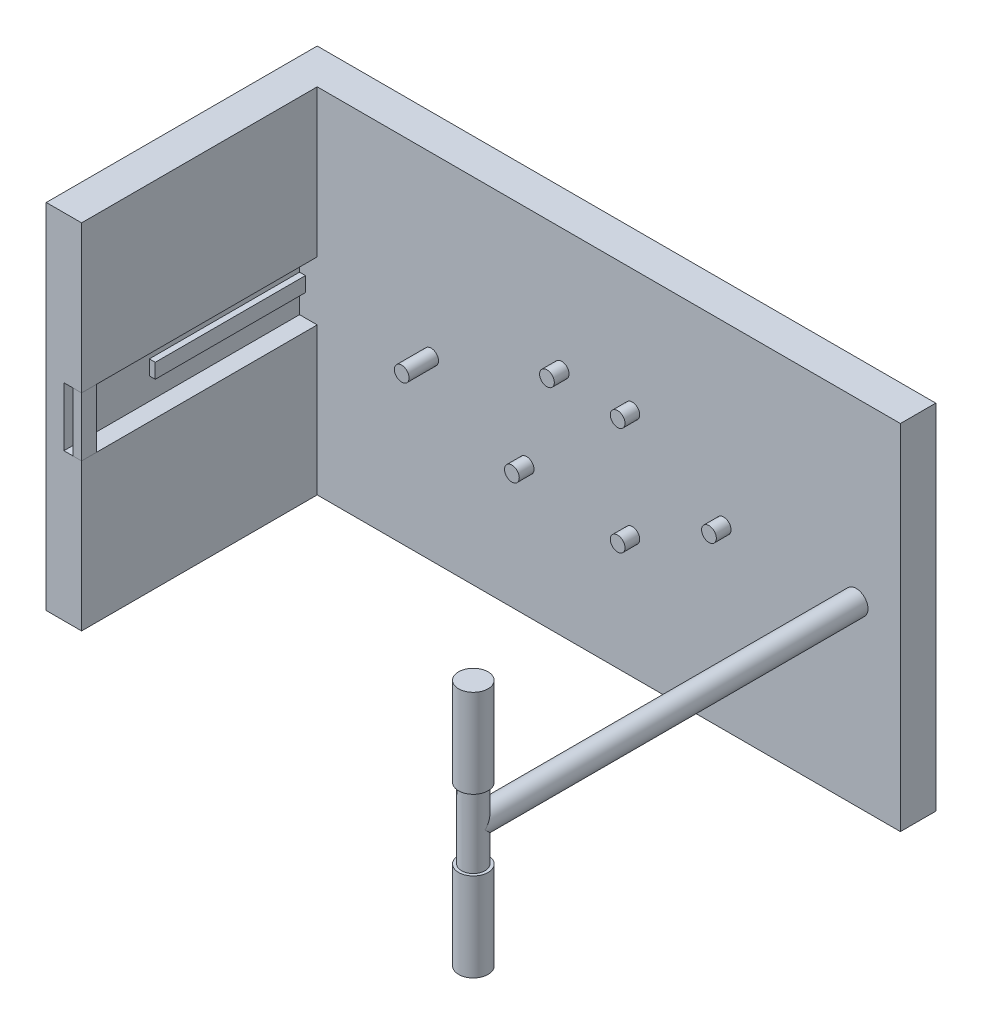
SolidWorks part; units mm, degrees
ref_plane "Front Plane" through (0, 0, 0) normal (0, 0, 1) x (1, 0, 0)
ref_plane "Top Plane" through (0, 0, 0) normal (0, 1, 0) x (1, 0, 0)
ref_plane "Right Plane" through (0, 0, 0) normal (1, 0, 0) x (0, 0, -1)
other "Configuration Table"
sketch "Sketch1" plane through (0, 0, 0) normal (0, 0, 1) x (1, 0, 0)
  line L0 (0, 3.2171) -> (0, -3.2171) construction
  point P4 (0, 0)
sketch "Sketch2" plane through (0, 0, 0) normal (0, 0, 1) x (1, 0, 0)
  line L1 (0, 0) -> (2100, 0)
  line L2 (0, 0) -> (0, -1200)
  line L3 (0, -1200) -> (2100, -1200)
  line L4 (2100, 0) -> (2100, -1200)
  dimension "D1" = 1200
  dimension "D2" = 2100
extrude "Boss-Extrude1" add sketch "Sketch2" along normal blind 120
sketch "Sketch3" plane through (0, 0, 120) normal (0, 0, 1) x (1, 0, 0)
  line L0 (0, -1200) -> (2100, -1200) construction
  line L1 (0, 0) -> (120, 0)
  line L2 (0, 0) -> (0, -1200)
  line L3 (0, -1200) -> (120, -1200)
  line L4 (120, 0) -> (120, -1200)
  dimension "D1" = 120
extrude "Boss-Extrude2" add sketch "Sketch3" along normal blind 800
sketch "Sketch4" plane through (0, 0, 120) normal (0, 0, 1) x (1, 0, 0)
  line L0 (1950, 0) -> (1950, -1200) construction
  line L1 (2100, 0) -> (120, 0) construction
  line L2 (120, -1200) -> (2100, -1200) construction
  line L3 (2100, -1200) -> (2100, 0) construction
  circle A0 centre (1950, -600) radius 40
  dimension "D2" = 80
  dimension "D1" = 150
extrude "Boss-Extrude3" add sketch "Sketch4" along normal blind 1300
sketch "Sketch5" plane through (0, 0, 1420) normal (0, 0, 1) x (1, 0, 0)
  line L0 (1950, -560) -> (1950, -640)
  line L1 (1990, -600) -> (1950, -600)
  circle A0 centre (1950, -600) radius 40 construction
  circle A1 centre (1950, -600) radius 40 construction
  dimension "D1" = 40
ref_plane "Plane1" through (0, -600, 0) normal (0, -1, 0) x (-1, 0, 0)
sketch "Sketch6" plane through (0, -600, 0) normal (0, -1, 0) x (-1, 0, 0)
  line L0 (-1990, -1420) -> (-1910, -1420) construction
  circle A0 centre (-1950, -1420) radius 40
  dimension "D1" = 80
extrude "Boss-Extrude4" add sketch "Sketch6" along normal blind 120 and the other way blind 120
sketch "Sketch7" plane through (0, -600, 0) normal (0, -1, 0) x (-1, 0, 0)
  circle A0 centre (-1950, -1420) radius 50
  dimension "D1" = 100
extrude "Boss-Extrude5" add sketch "Sketch7" along normal blind 300 from offset 120
mirror "Mirror1" about plane through (0, -600, 0) normal (0, -1, 0) of "Boss-Extrude5"
sketch "Sketch9" plane through (0, 0, 120) normal (0, 0, 1) x (1, 0, 0)
  line L0 (2100, -600) -> (1500, -600)
  line L1 (2100, -1200) -> (2100, 0) construction
  circle A0 centre (1500, -600) radius 250 construction
  circle A1 centre (1500, -600) radius 25
  dimension "D1" = 500
  dimension "D3" = 50
  dimension "D2" = 600
extrude "Boss-Extrude6" add sketch "Sketch9" along normal blind 50
sketch "Sketch10" plane through (0, 0, 120) normal (0, 0, 1) x (1, 0, 0)
  line L0 (1500, -600) -> (1190, -600) construction
  line L1 (1190, -416.9699) -> (1190, -783.0301) construction
  line L2 (2100, -600) -> (1500, -600) construction
  circle A0 centre (1500, -600) radius 360 construction
  circle A1 centre (1190, -416.9699) radius 25
  circle A2 centre (1190, -783.0301) radius 25
  dimension "D2" = 50
  dimension "D3" = 50
  dimension "D4" = 720
  dimension "D1" = 310
extrude "Boss-Extrude7" add sketch "Sketch10" along normal blind 50
sketch "Sketch11" plane through (0, 0, 120) normal (0, 0, 1) x (1, 0, 0)
  line L0 (1190, -416.9699) -> (950, -416.9699) construction
  circle A0 centre (950, -416.9699) radius 25
  dimension "D1" = 50
  dimension "D2" = 240
extrude "Boss-Extrude8" add sketch "Sketch11" along normal blind 50
sketch "Sketch12" plane through (0, 0, 120) normal (0, 0, 1) x (1, 0, 0)
  line L1 (2100, -1200) -> (2100, 0) construction
  line L2 (120, -1200) -> (2100, -1200) construction
  circle A0 centre (830.9627, -756.72) radius 25
  dimension "D3" = 50
  dimension "D1" = 443.28
  dimension "D2" = 1269.0373
extrude "Boss-Extrude9" add sketch "Sketch12" along normal blind 50
sketch "Sketch13" plane through (0, 0, 120) normal (0, 0, 1) x (1, 0, 0)
  line L0 (2100, -600) -> (120, -600) construction
  line L1 (2100, -1200) -> (2100, 0) construction
  line L2 (120, -1200) -> (120, 0) construction
  line L3 (830.9627, -756.72) -> (506.8658, -600) construction
  circle A0 centre (506.8658, -600) radius 25
  dimension "D2" = 50
  dimension "D1" = 360
extrude "Boss-Extrude10" add sketch "Sketch13" along normal blind 100
sketch "Sketch14" plane through (0, 0, 920) normal (0, 0, 1) x (1, 0, 0)
  line L0 (120, -600) -> (0, -600) construction
  line L1 (120, -1200) -> (120, 0) construction
  line L2 (0, 0) -> (0, -1200) construction
  line L4 (180, -500) -> (60, -500)
  line L5 (180, -500) -> (180, -700)
  line L6 (180, -700) -> (60, -700)
  line L7 (60, -500) -> (60, -700)
  line L8 (120, -700) -> (120, -500) construction
  line L9 (180, -600) -> (60, -600) construction
  dimension "D1" = 60
  dimension "D2" = 200
extrude "Cut-Extrude1" cut sketch "Sketch14" against normal up to surface (800 mm away) up to face at (531.8658, -600, 120)
sketch "Sketch15" plane through (60, 0, 0) normal (1, 0, 0) x (0, 0, -1)
  line L0 (-120, -600) -> (-630, -600) construction
  line L1 (-120, -700) -> (-120, -500) construction
  line L4 (-120, -575) -> (-630, -575)
  line L5 (-120, -575) -> (-120, -625)
  line L6 (-120, -625) -> (-630, -625)
  line L7 (-630, -575) -> (-630, -625)
  line L8 (-375, -625) -> (-375, -575) construction
  line L9 (-120, -600) -> (-630, -600) construction
  point P5 (-375, -600)
  dimension "D1" = 510
  dimension "D2" = 50
extrude "Boss-Extrude11" add sketch "Sketch15" along normal blind 20
sketch "Sketch16" plane through (0, -500, 0) normal (0, -1, 0) x (1, 0, 0)
  line L1 (120, 920) -> (90, 920)
  line L2 (120, 920) -> (120, 870)
  line L3 (120, 870) -> (90, 870)
  line L4 (90, 920) -> (90, 870)
  dimension "D1" = 30
  dimension "D2" = 50
extrude "Boss-Extrude12" add sketch "Sketch16" along normal blind 200 separate body
